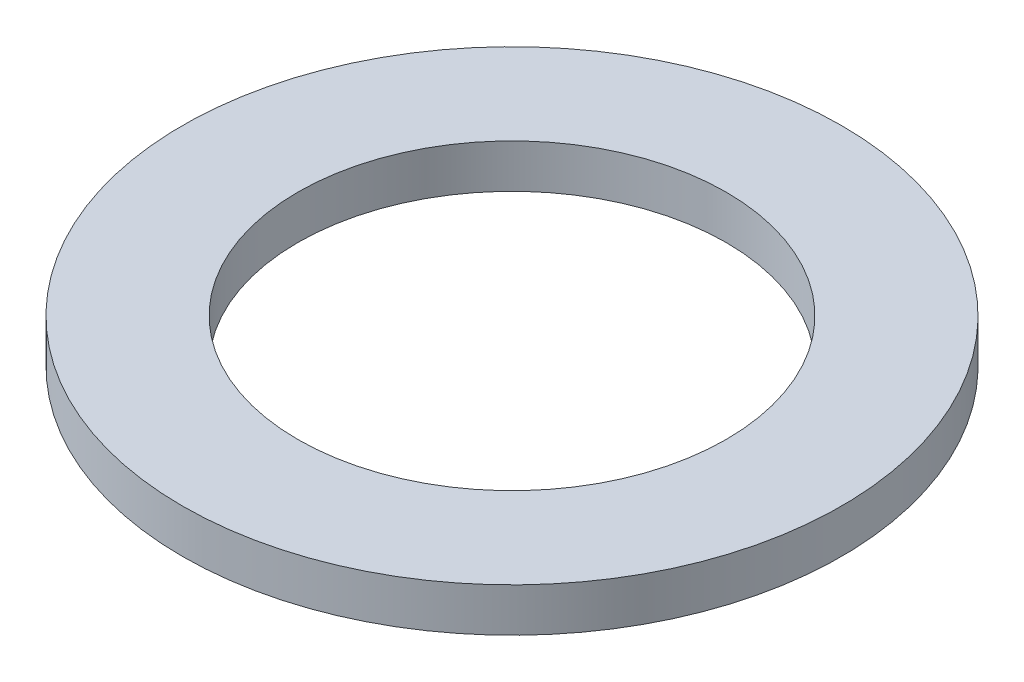
SolidWorks part; units mm, degrees
ref_plane "Front Plane" through (0, 0, 0) normal (0, 0, 1) x (1, 0, 0)
ref_plane "Top Plane" through (0, 0, 0) normal (0, 1, 0) x (1, 0, 0)
ref_plane "Right Plane" through (0, 0, 0) normal (1, 0, 0) x (0, 0, -1)
other "Configuration Table"
sketch "Sketch1" plane through (0, 0, 0) normal (0, 1, 0) x (1, 0, 0)
  circle A0 centre (0, 0) radius 26
  circle A1 centre (0, 0) radius 40
  dimension "D1" = 52
  dimension "D2" = 80
extrude "Boss-Extrude1" add sketch "Sketch1" along normal blind 5.3
